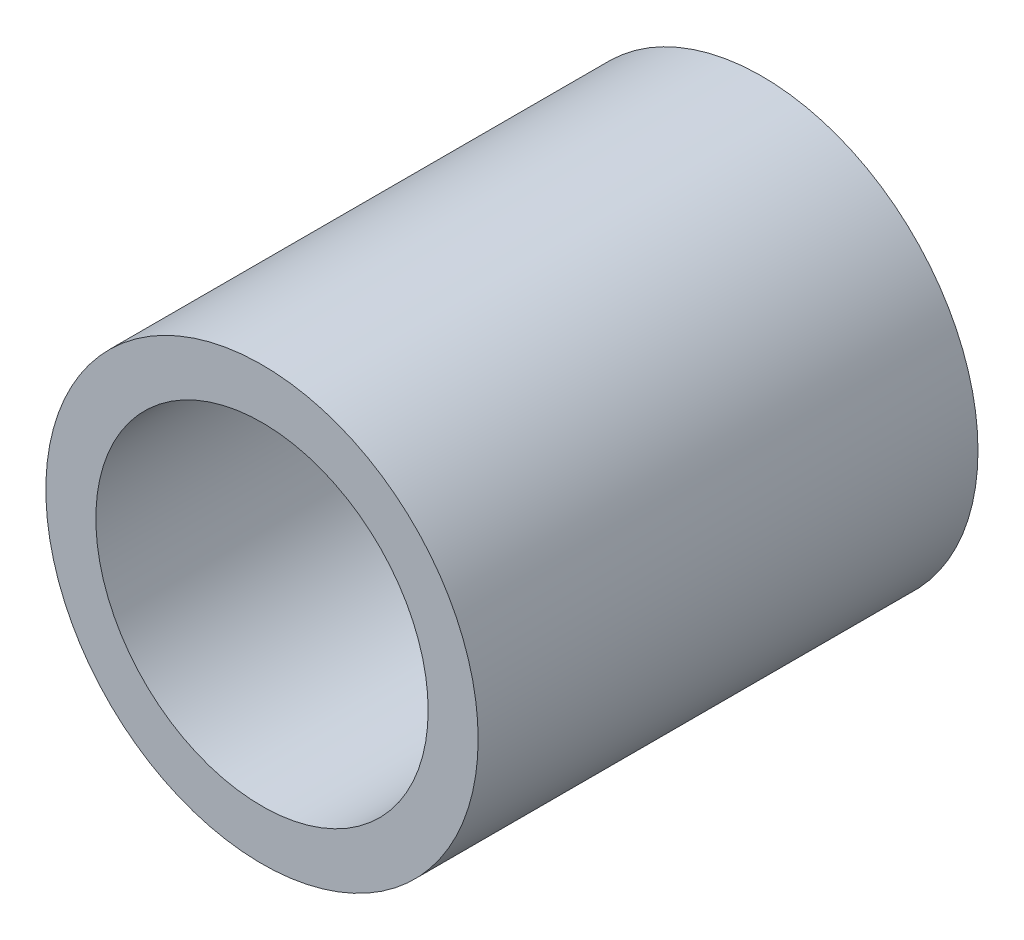
SolidWorks part; units mm, degrees
ref_plane "Front Plane" through (0, 0, 0) normal (0, 0, 1) x (1, 0, 0)
ref_plane "Top Plane" through (0, 0, 0) normal (0, 1, 0) x (1, 0, 0)
ref_plane "Right Plane" through (0, 0, 0) normal (1, 0, 0) x (0, 0, -1)
sketch "Sketch1" plane through (0, 0, 0) normal (0, 0, 1) x (1, 0, 0)
  circle A0 centre (100, 71.3) radius 6.15
  circle A1 centre (100, 71.3) radius 8
  dimension "D1" = 12.3
  dimension "D2" = 16
extrude "Boss-Extrude1" add sketch "Sketch1" along normal up to surface (18.5 mm away)
